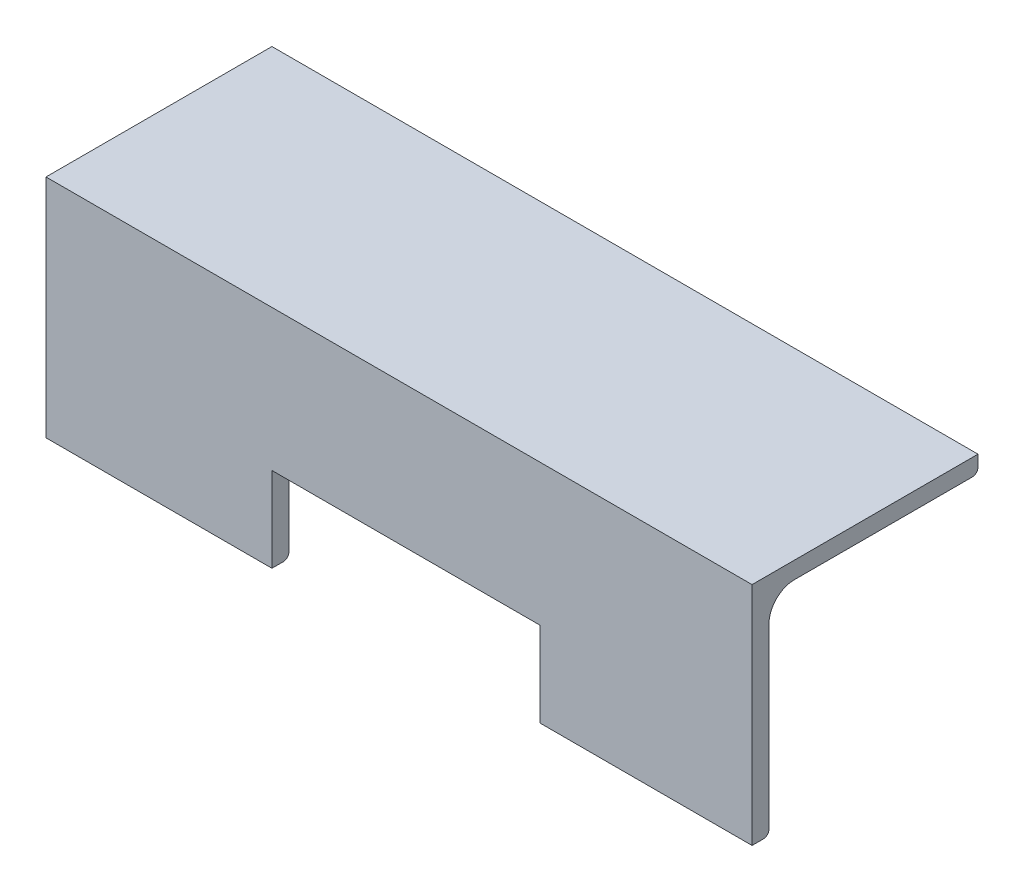
SolidWorks part; units mm, degrees
material "Q235-A"
ref_plane "Front Plane" through (0, 0, 0) normal (0, 0, 1) x (1, 0, 0)
ref_plane "Top Plane" through (0, 0, 0) normal (0, 1, 0) x (1, 0, 0)
ref_plane "Right Plane" through (0, 0, 0) normal (1, 0, 0) x (0, 0, -1)
sketch "草图1" plane through (0, 0, 0) normal (0, 0, 1) x (1, 0, 0)
  line L0 (125, 0) -> (-125, 0)
  point P4 (0, 0)
  dimension "D1" = 250
other "hot-rolled equal angle steel (GB/T 9787-1988) 80×6(1)"
ref_plane "Plane1" through (125, 0, 0) normal (-1, 0, 0) x (0, -1, 0)
sketch "Sketch1" plane through (125, 0, 0) normal (-1, 0, 0) x (0, -1, 0)
  line L0 (80, 0) -> (0, 0)
  line L1 (0, 0) -> (0, -80)
  line L2 (78, -6) -> (15, -6)
  line L3 (6, -15) -> (6, -78)
  line L4 (80, 0) -> (80, -4)
  line L5 (0, -80) -> (4, -80)
  arc A0 (80, -4) -> (78, -6) centre (78, -4) cw
  arc A1 (4, -80) -> (6, -78) centre (4, -78) ccw
  arc A2 (15, -6) -> (6, -15) centre (15, -15) ccw
  point P2 (40, 0)
  point P13 (0, -40)
  point P15 (0, 0)
  dimension "r1" = 2
  dimension "r" = 9
  dimension "b" = 80
  dimension "d" = 6
sketch "Sketch3" plane through (0, 0, -6) normal (0, 0, -1) x (-1, 0, 0)
  line L0 (45, -99.5199) -> (45, -50)
  line L1 (45, -50) -> (-50, -50)
  line L2 (-50, -50) -> (-50, -99.5199)
  line L3 (45, -99.5199) -> (-50, -99.5199)
  line L4 (125, -15) -> (125, -78) construction
  line L5 (125, -80) -> (-125, -80) construction
  dimension "D1" = 80
  dimension "D2" = 95
  dimension "D3" = 30
extrude "Cut-Extrude1" cut sketch "Sketch3" against normal blind 10
